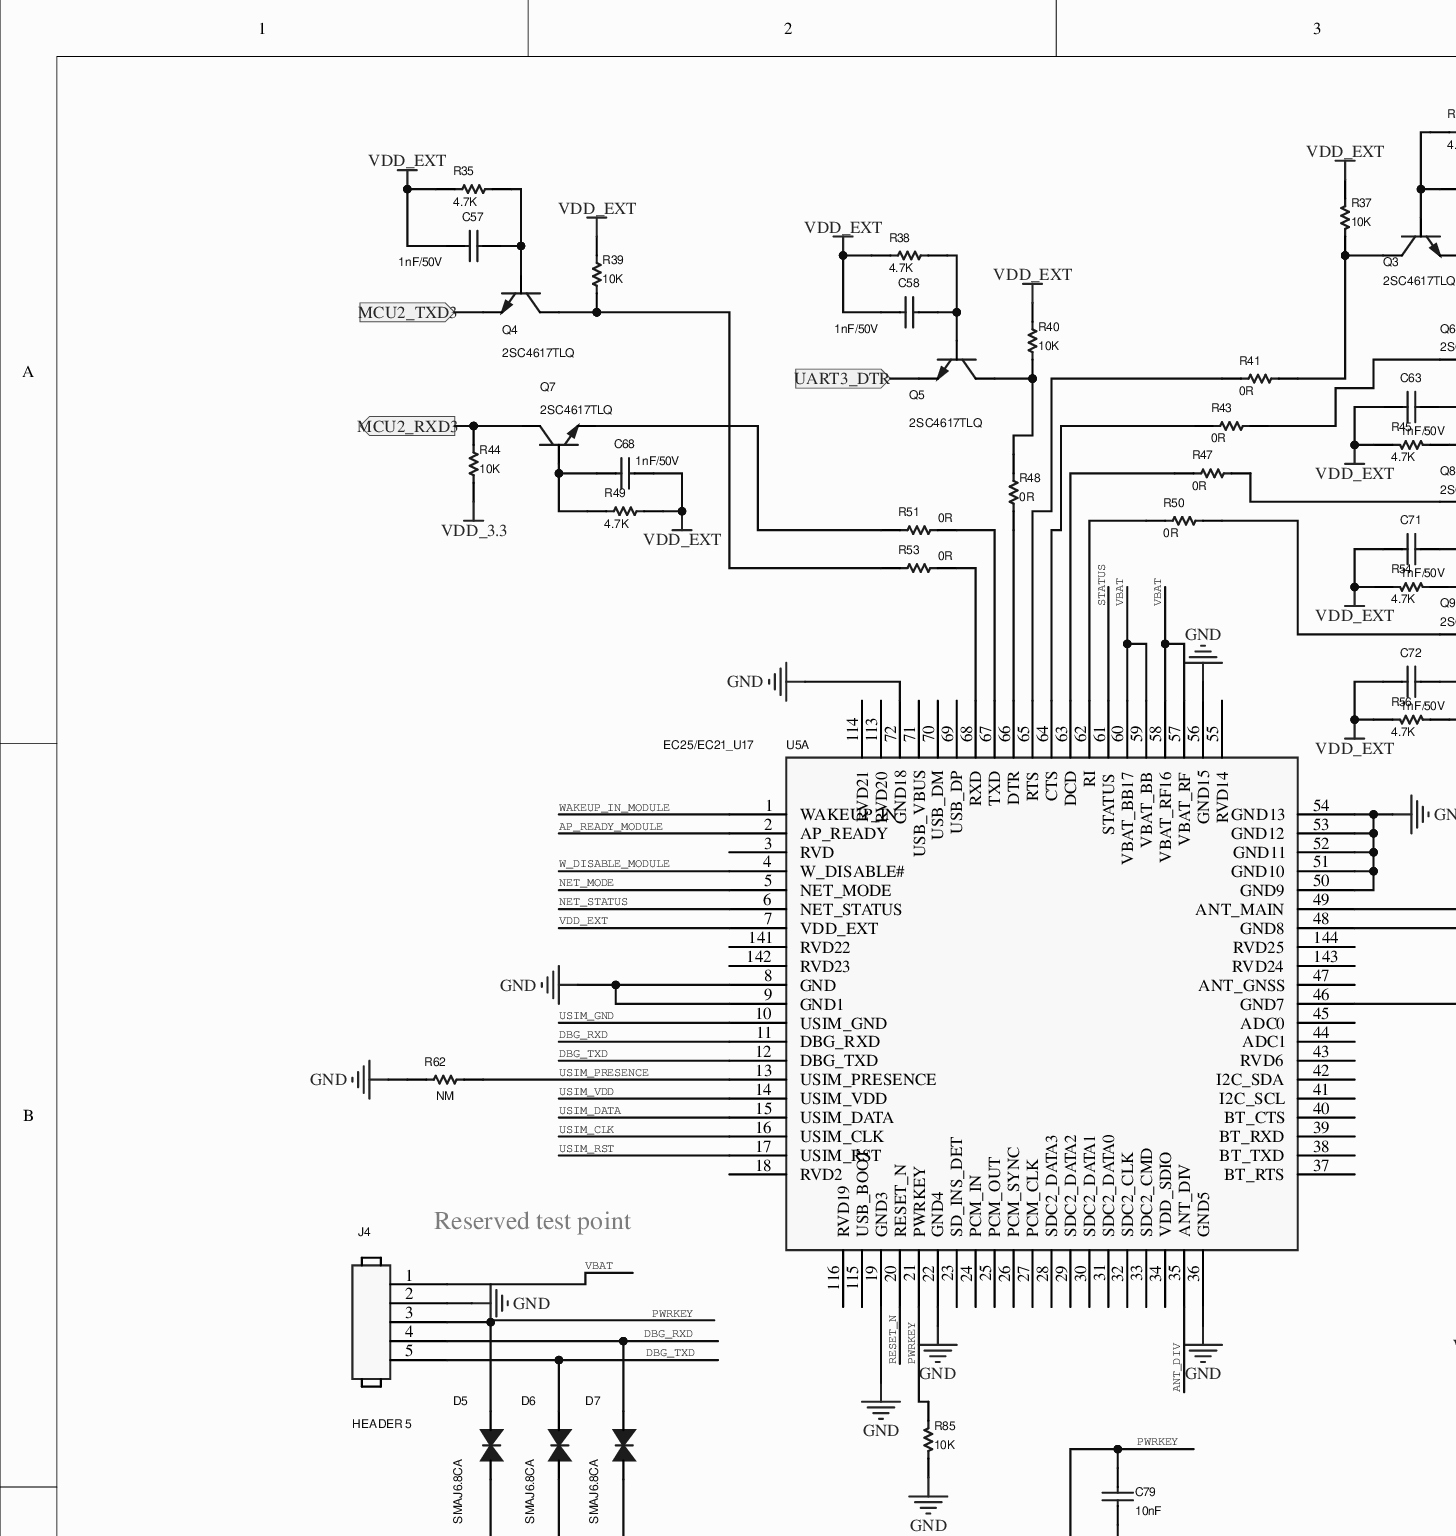
[diagram p0: MISC86294-12.SchDoc, top left]
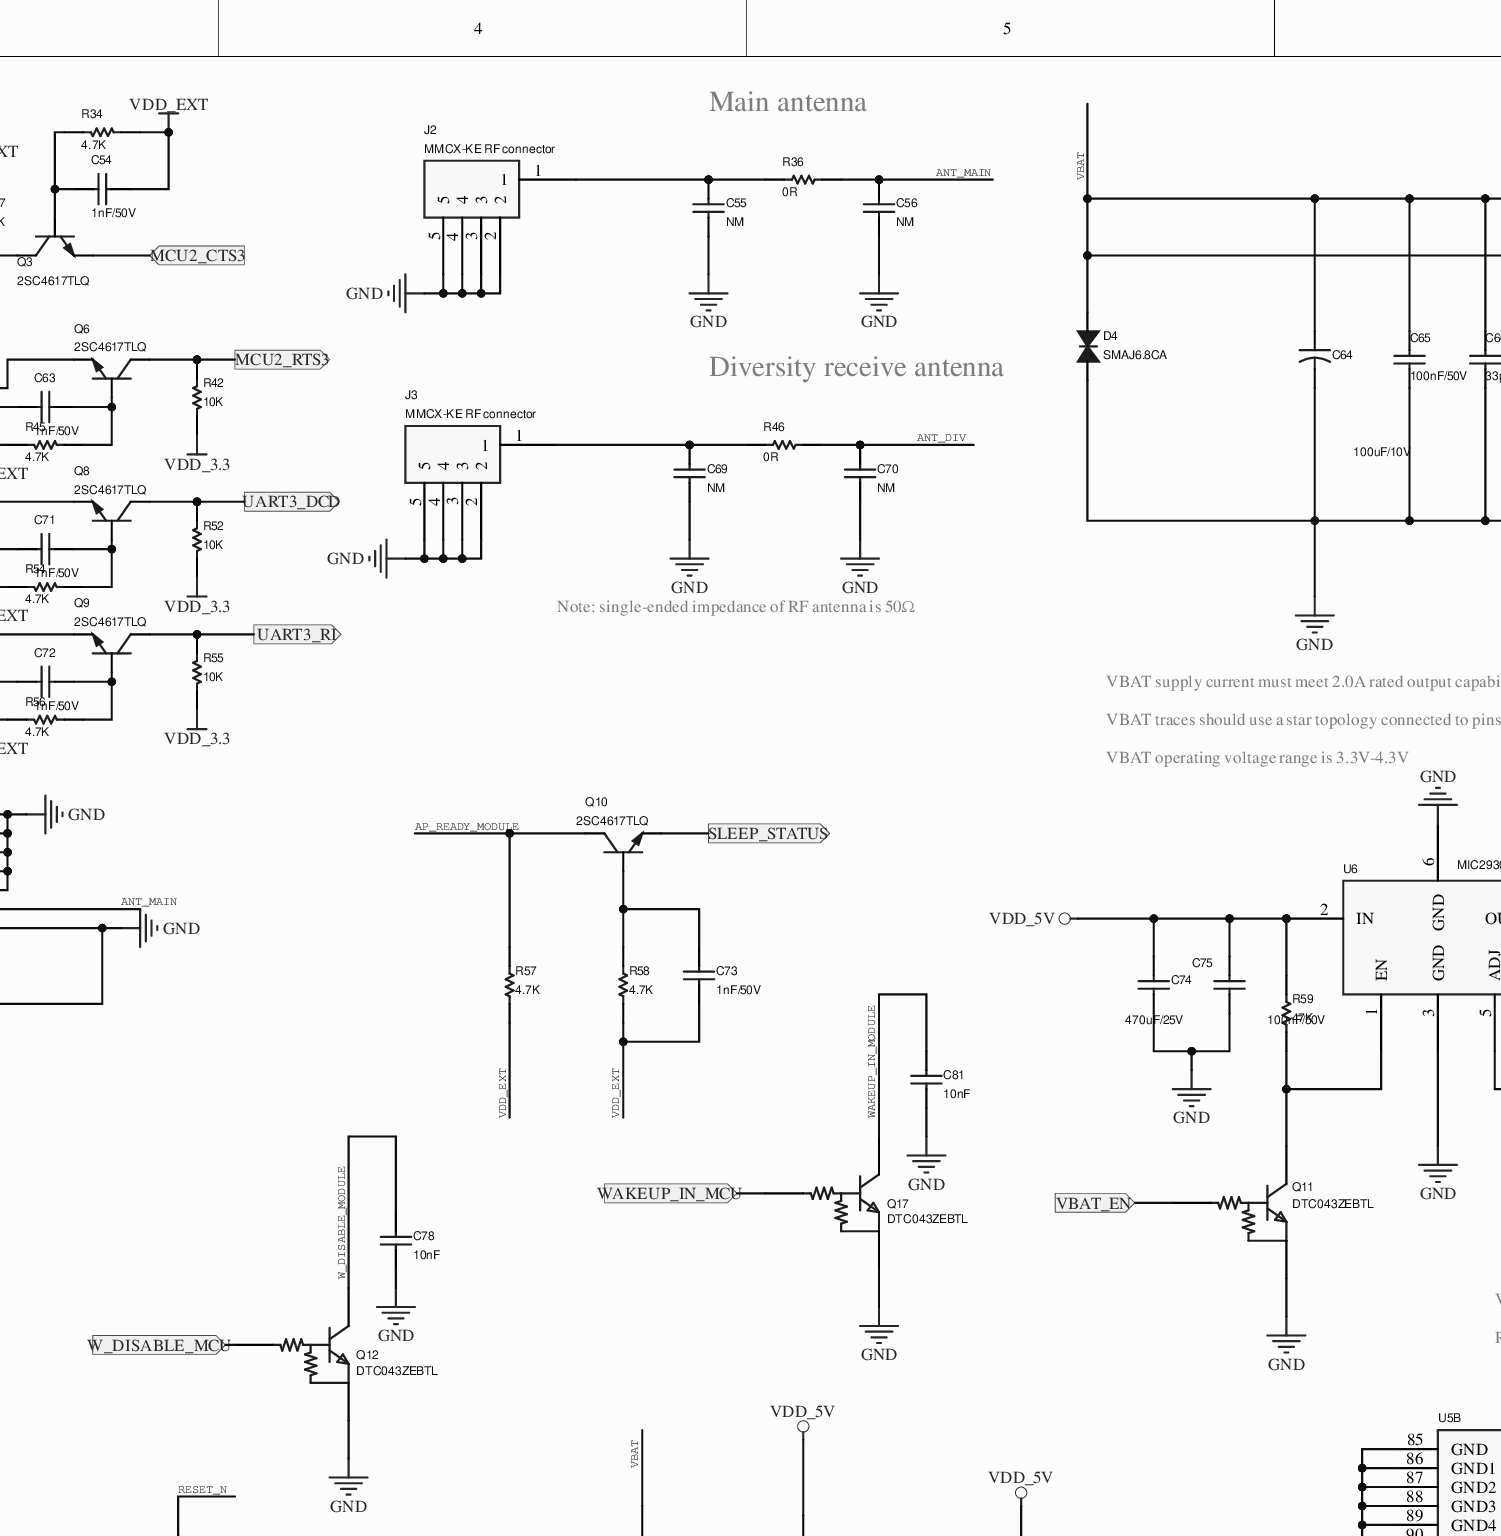
[diagram p1: MISC86294-12.SchDoc, top middle]
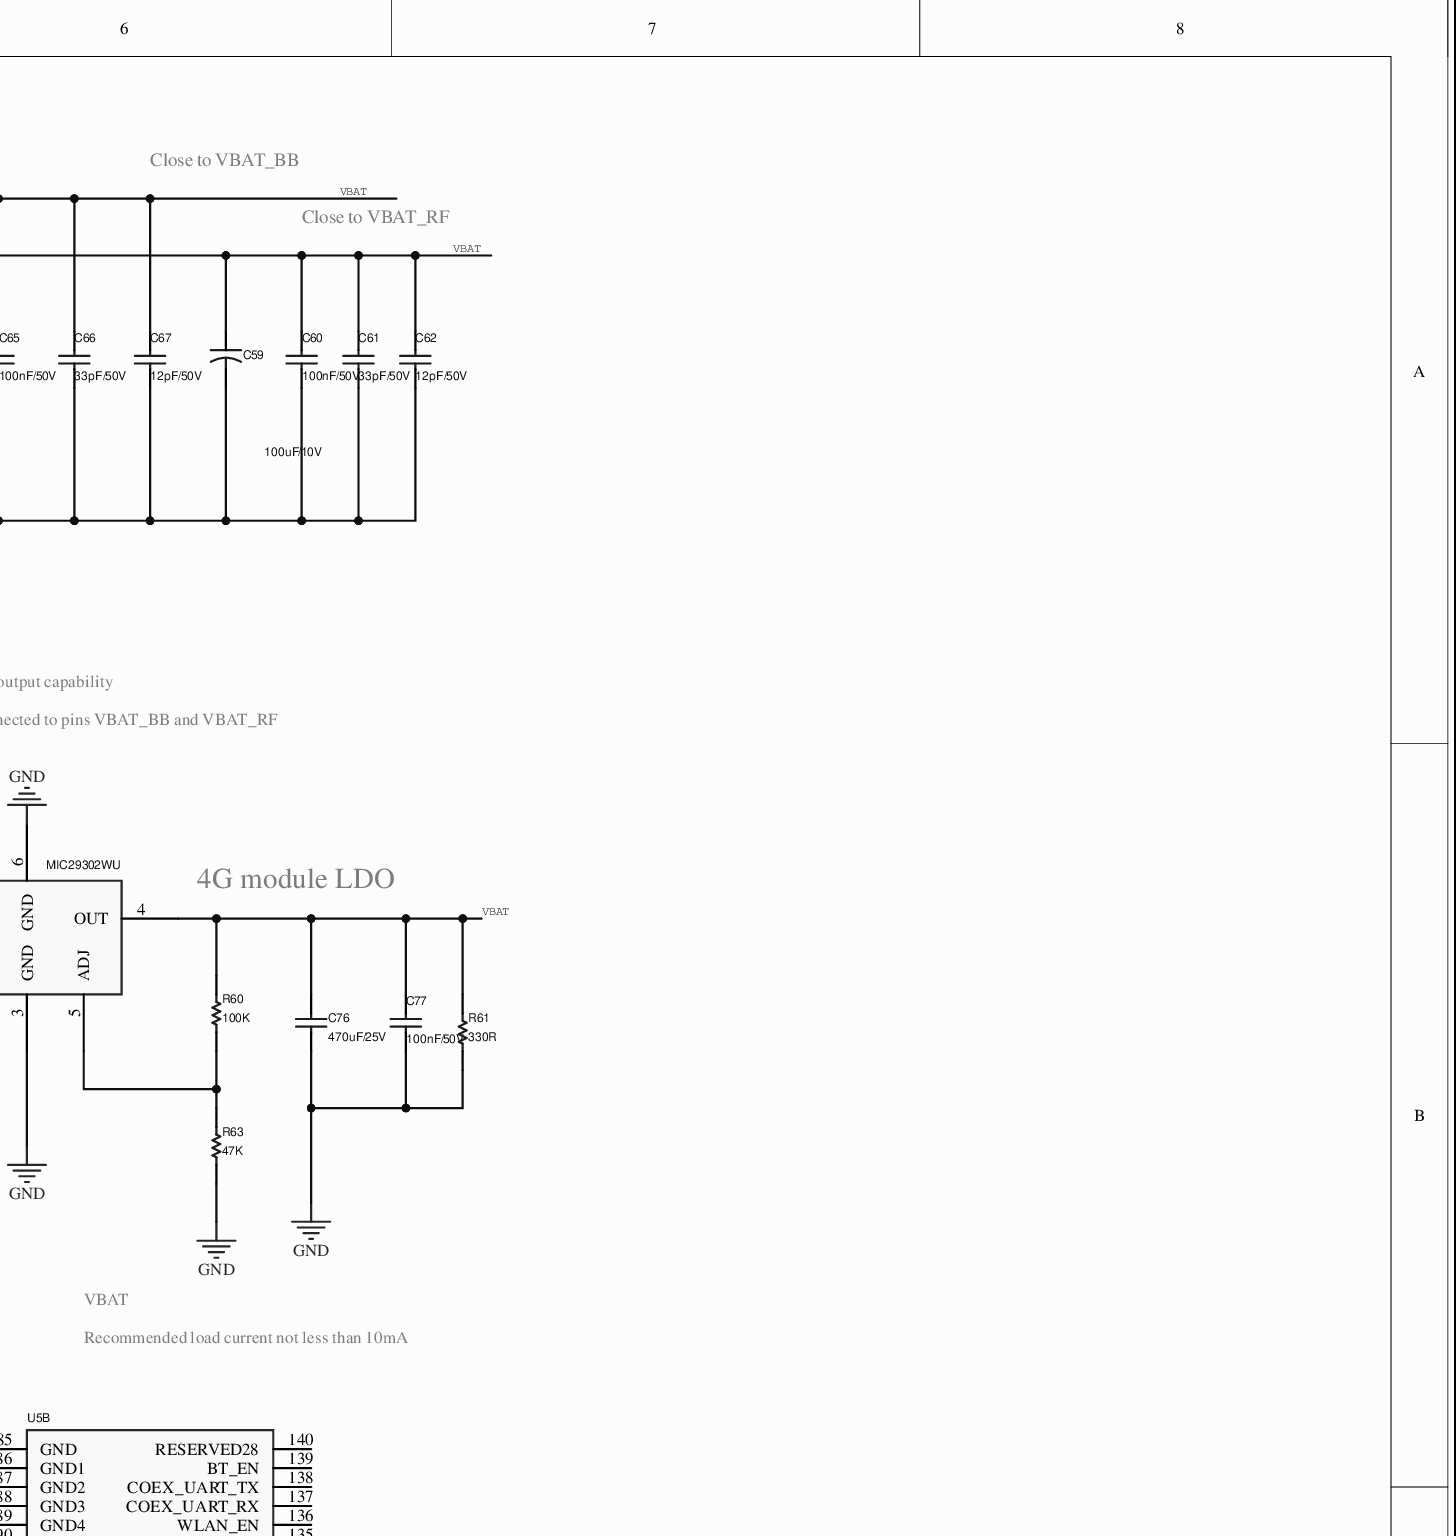
[diagram p2: MISC86294-12.SchDoc, top right]
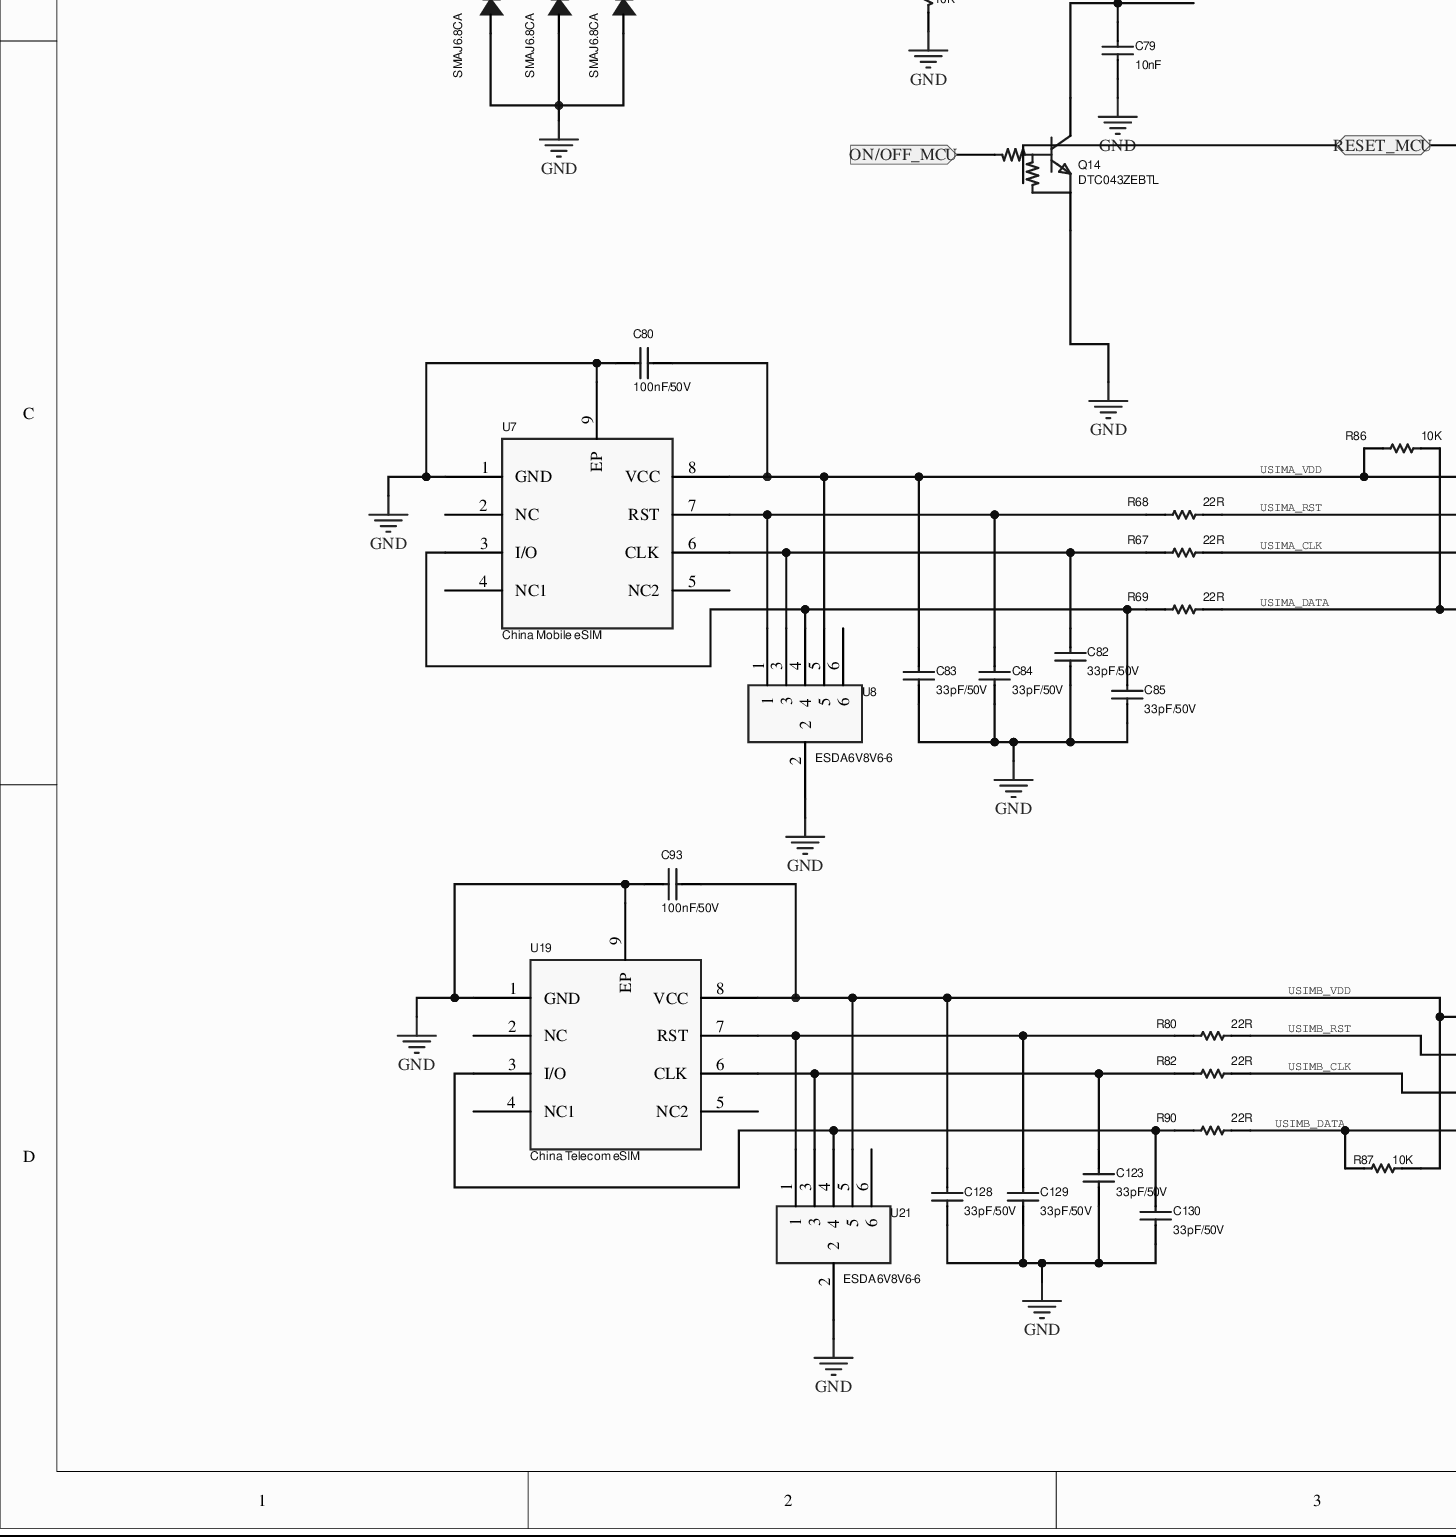
[diagram p3: MISC86294-12.SchDoc, bottom left]
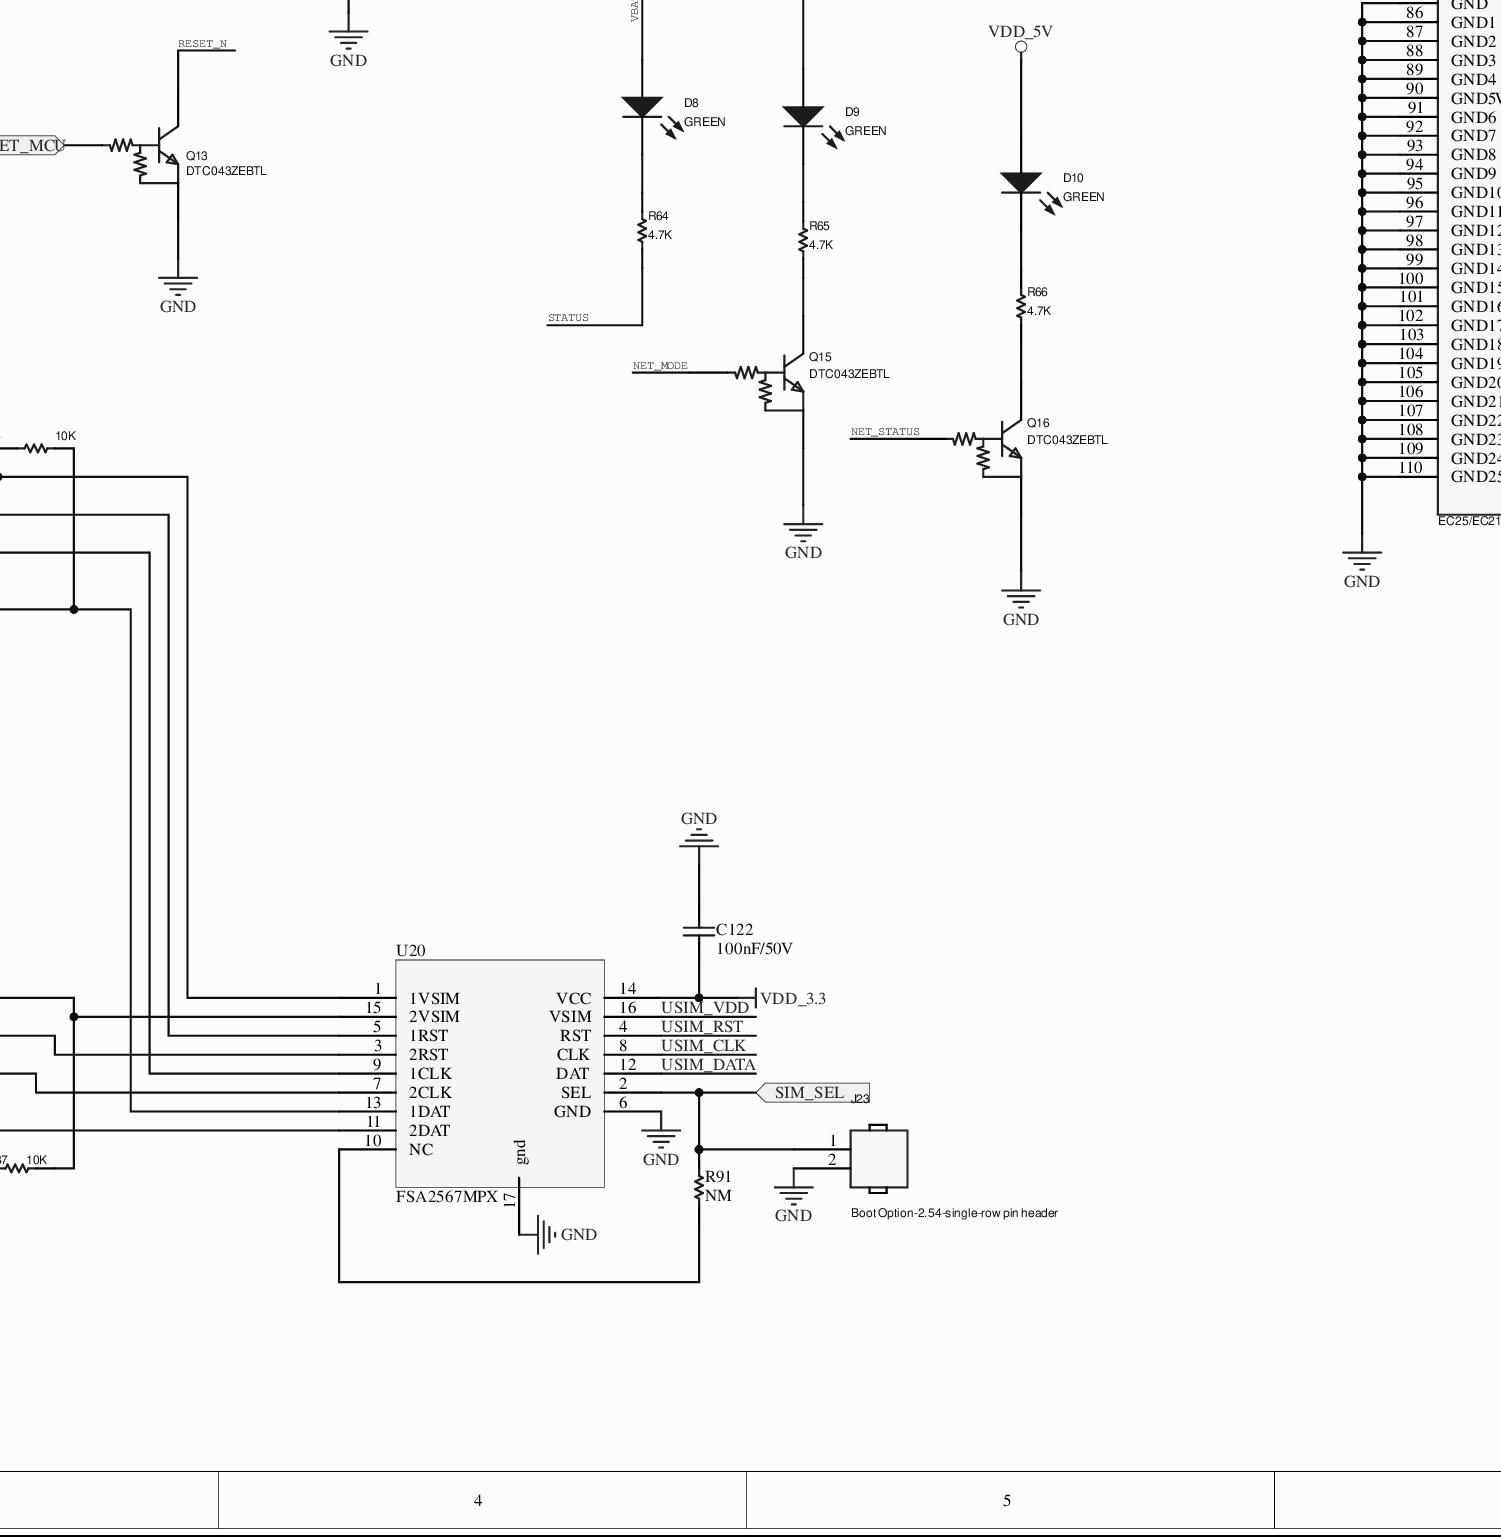
[diagram p4: MISC86294-12.SchDoc, bottom middle]
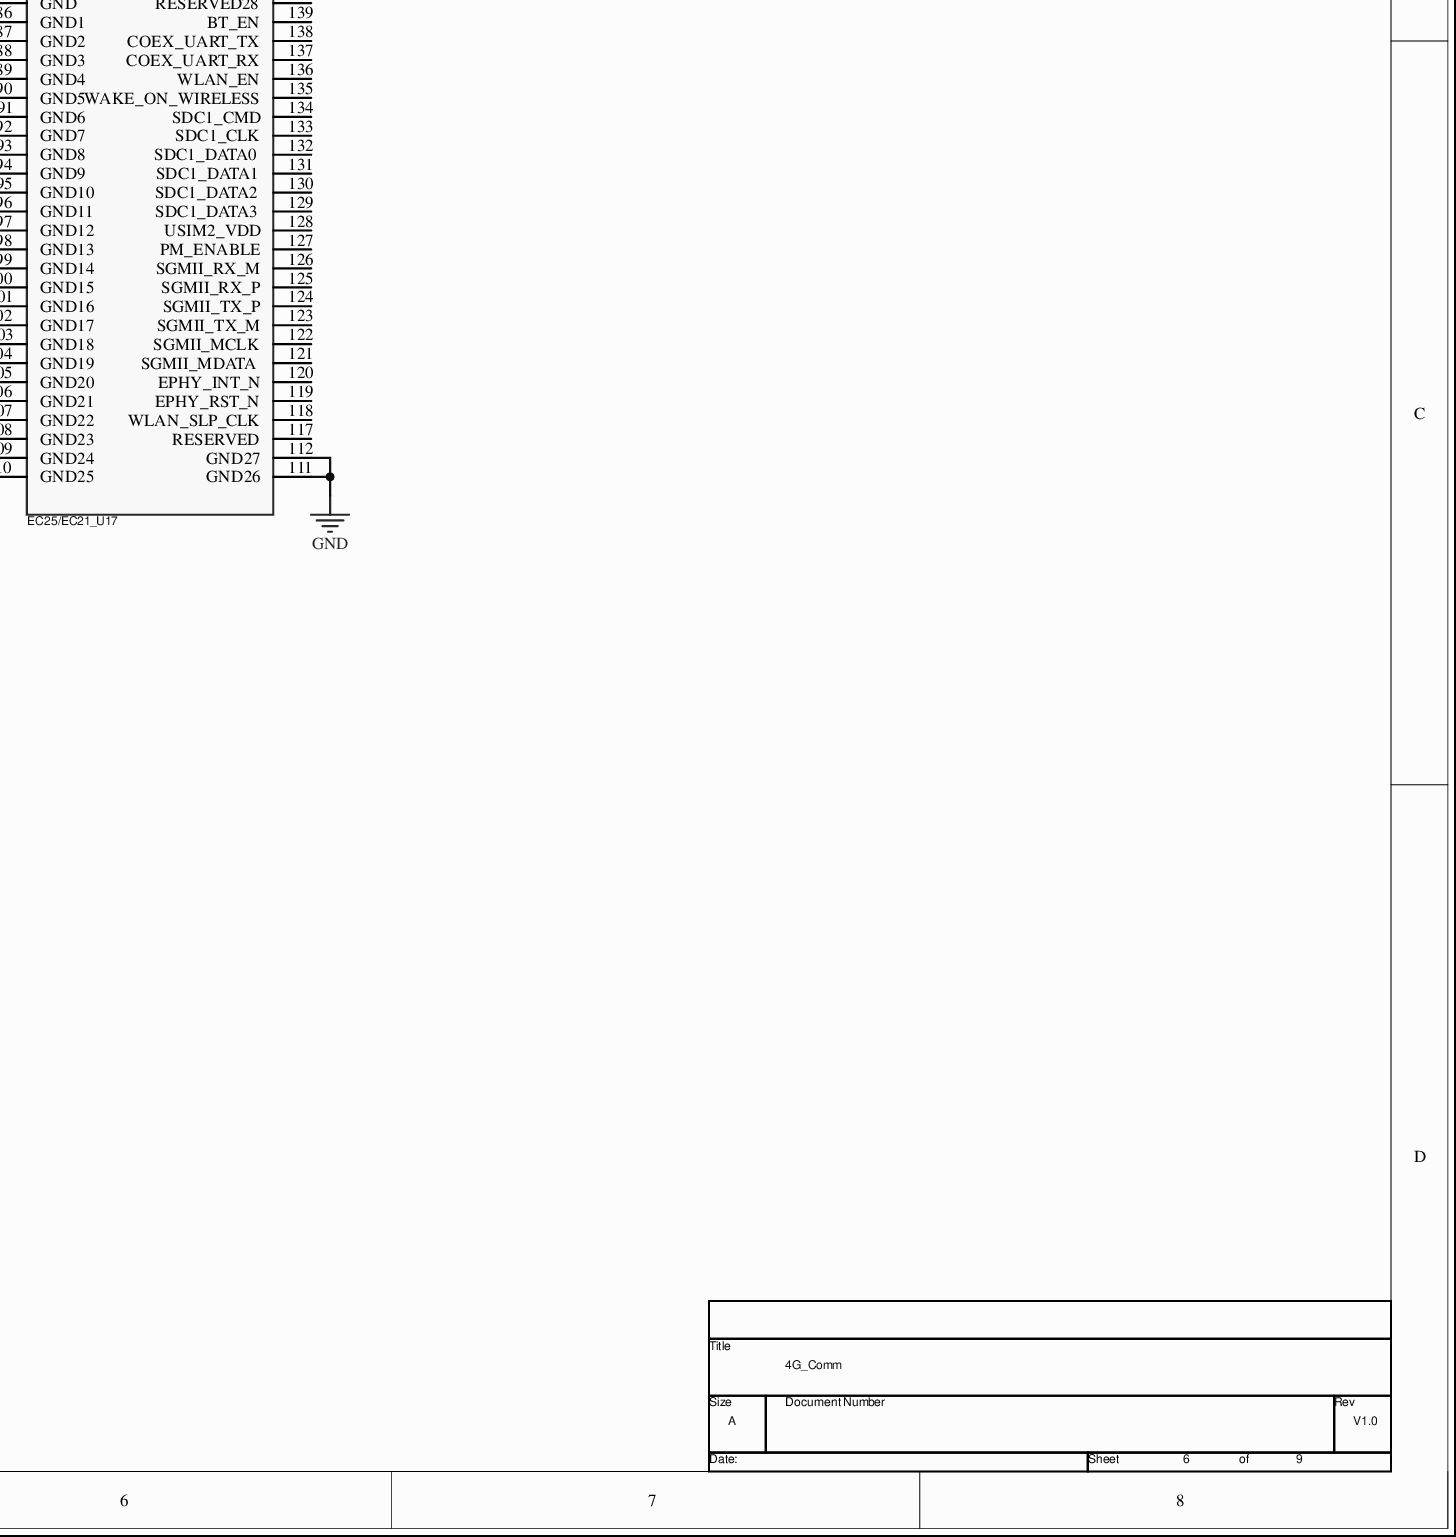
[diagram p5: MISC86294-12.SchDoc, bottom right]
# Altium project MISC86294-22.PrjPcb (part 3 of 5)
## Sheet MISC86294-12.SchDoc
size A2

### Parts
(Parts that share a designator on the sheet are numbered #1, #2 ... from top to bottom, then left to right.)
*#5  RevCode: V1.0  Title: 4G_Comm  Page Size: A  Page Number: 6  Page Count: 9  (hidden comment: TitleBlock0)  (graphical)
C54  1nF/50V  [C0603]
C55  NM  [C0603]
C56  NM  [C0603]
C57  1nF/50V  [C0603]
C58  1nF/50V  [C0603]
C59  100uF/10V  [RB5*7]
C60  100nF/50V  [C0603]
C61  33pF/50V  [C0603]
C62  12pF/50V  [C0603]
C63  1nF/50V  [C0603]
C64  100uF/10V  [RB5*7]
C65  100nF/50V  [C0603]
C66  33pF/50V  [C0603]
C67  12pF/50V  [C0603]
C68  1nF/50V  [C0603]
C69  NM  [C0603]
C70  NM  [C0603]
C71  1nF/50V  [C0603]
C72  1nF/50V  [C0603]
C73  1nF/50V  [C0603]
C74  470uF/25V  [RB8*11_5]
C75  100nF/50V  [C0603]
C76  470uF/25V  [RB8*11_5]
C77  100nF/50V  [C0603]
C78  10nF  [C0603]
C79  10nF  [C0603]
C80  100nF/50V  [C0603]